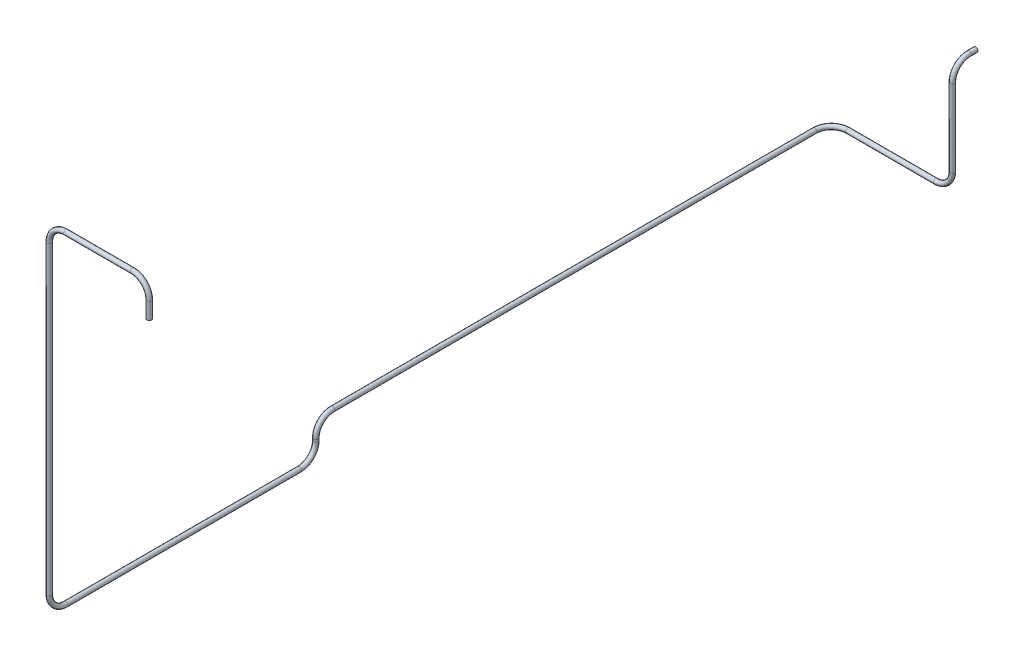
from build123d import *

# Parameters (mm, degrees)
SKETCH_2_R    = 7
SKETCH_2_R_2  = 4
SKETCH_4_R    = 7
SKETCH_4_R_2  = 4
SKETCH_6_R    = 7
SKETCH_6_R_2  = 4
SKETCH_8_R    = 7
SKETCH_8_R_2  = 4
SKETCH_10_R   = 7
SKETCH_10_R_2 = 4


with BuildPart() as part:
    # Sweep 1: sweep along a path in Sketch 1
    with BuildLine(Plane.XY) as sweep_1_path:
        Line((150, 0), (150, 50))
        ThreePointArc((150, 50), (135.355339059, 85.355339059), (100, 100))
        Line((100, 100), (-100, 100))
        ThreePointArc((-100, 100), (-135.355339059, 85.355339059), (-150, 50))
        Line((-150, 50), (-150, -816.5))
    # Sketch 2 → Sweep 1 (sweep)
    with BuildSketch(Plane(origin=(0, 0, 0), x_dir=(1, 0, 0), z_dir=(0, 1, 0))):
        with Locations((150, 0)):
            Circle(SKETCH_2_R)
        with Locations((150, 0)):
            Circle(SKETCH_2_R_2, mode=Mode.SUBTRACT)
    sweep(path=sweep_1_path.line)

    # Sweep 2: sweep along a path in Sketch 3
    with BuildLine(Plane(origin=(-150, 0, 0), x_dir=(0, 0, -1), z_dir=(1, 0, 0))) as sweep_2_path:
        Line((0, -816.5), (0, -866.5))
        ThreePointArc((0, -866.5), (14.644660941, -901.855339059), (50, -916.5))
        Line((50, -916.5), (750, -916.5))
        ThreePointArc((750, -916.5), (785.355339059, -901.855339059), (800, -866.5))
        Line((800, -866.5), (800, -859.5))
        ThreePointArc((800, -859.5), (814.644660941, -824.144660941), (850, -809.5))
        Line((850, -809.5), (2247.5, -809.5))
    # Sketch 4 → Sweep 2 (sweep)
    with BuildSketch(Plane.XZ.offset(816.5)):
        with Locations((-150, 0)):
            Circle(SKETCH_4_R)
        with Locations((-150, 0)):
            Circle(SKETCH_4_R_2, mode=Mode.SUBTRACT)
    sweep(path=sweep_2_path.line)

    # Sweep 3: sweep along a path in Sketch 5
    with BuildLine(Plane(origin=(0, -809.5, 0), x_dir=(1, 0, 0), z_dir=(0, 1, 0))) as sweep_3_path:
        Line((-150, 2247.5), (-150, 2297.5))
        ThreePointArc((-150, 2297.5), (-135.355339059, 2332.855339059), (-100, 2347.5))
        Line((-100, 2347.5), (113.2, 2347.5))
    # Sketch 6 → Sweep 3 (sweep)
    with BuildSketch(Plane(origin=(0, 0, -2247.5), x_dir=(-1, 0, 0), z_dir=(0, 0, -1))):
        with Locations((150, -809.5)):
            Circle(SKETCH_6_R)
        with Locations((150, -809.5)):
            Circle(SKETCH_6_R_2, mode=Mode.SUBTRACT)
    sweep(path=sweep_3_path.line)

    # Sweep 4: sweep along a path in Sketch 7
    with BuildLine(Plane.XY.offset(-2347.5)) as sweep_4_path:
        Line((113.2, -809.5), (163.2, -809.5))
        ThreePointArc((163.2, -809.5), (198.555339059, -794.855339059), (213.2, -759.5))
        Line((213.2, -759.5), (213.2, -577.5))
    # Sketch 8 → Sweep 4 (sweep)
    with BuildSketch(Plane(origin=(113.2, 0, 0), x_dir=(0, 0, -1), z_dir=(1, 0, 0))):
        with Locations((2347.5, -809.5)):
            Circle(SKETCH_8_R)
        with Locations((2347.5, -809.5)):
            Circle(SKETCH_8_R_2, mode=Mode.SUBTRACT)
    sweep(path=sweep_4_path.line)

    # Sweep 5: sweep along a path in Sketch 9
    with BuildLine(Plane(origin=(213.2, 0, 0), x_dir=(0, 0, -1), z_dir=(1, 0, 0))) as sweep_5_path:
        Line((2347.5, -577.5), (2347.5, -527.5))
        ThreePointArc((2347.5, -527.5), (2362.144660941, -492.144660941), (2397.5, -477.5))
        Line((2397.5, -477.5), (2417.5, -477.5))
    # Sketch 10 → Sweep 5 (sweep)
    with BuildSketch(Plane(origin=(0, -577.5, 0), x_dir=(1, 0, 0), z_dir=(0, 1, 0))):
        with Locations((213.2, 2347.5)):
            Circle(SKETCH_10_R)
        with Locations((213.2, 2347.5)):
            Circle(SKETCH_10_R_2, mode=Mode.SUBTRACT)
    sweep(path=sweep_5_path.line)


solid = part.part
